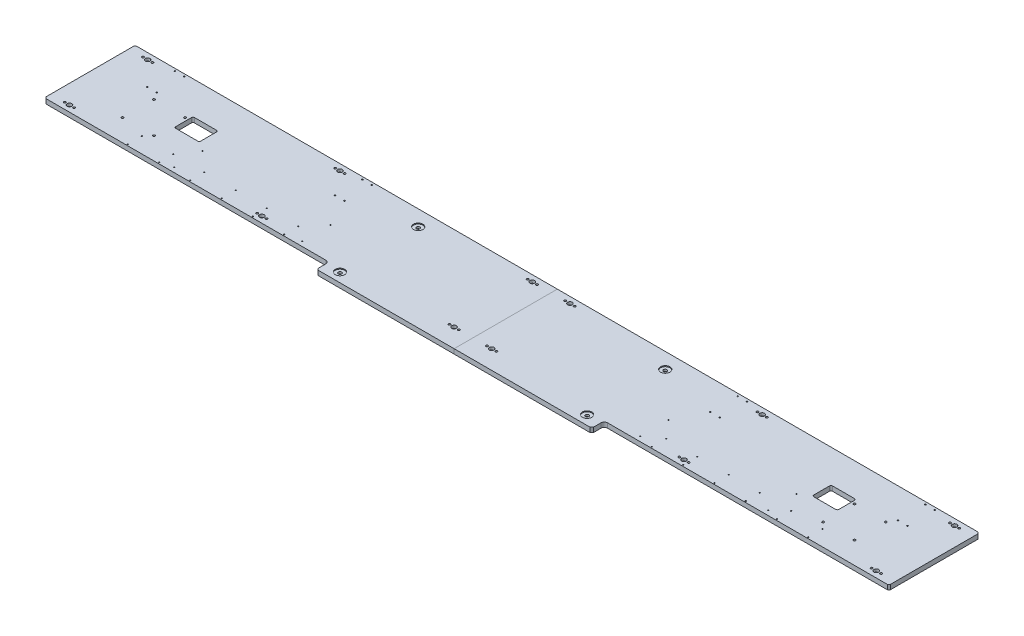
from build123d import *

# Parameters (mm, degrees)
SKETCH_1_W                = 2700
SKETCH_1_H                = 290
EXTRUDE_1_DEPTH           = 20
SKETCH_18_W               = 880
SKETCH_18_H               = 40
EXTRUDE_2_DEPTH           = 20
CHAMFER_1_SIZE            = 5
HOLE_WIZARD_1_D           = 9
HOLE_WIZARD_1_CBORE_D     = 15
HOLE_WIZARD_1_CBORE_DEPTH = 9
HOLE_WIZARD_M5_1_D        = 4.2
HOLE_WIZARD_M5_1_DEPTH    = 12.4
HOLE_WIZARD_M5_1_TIP      = 1.2618073
HOLE_WIZARD_M4_1_D        = 3.3
HOLE_WIZARD_M4_1_DEPTH    = 10.1
HOLE_WIZARD_M4_1_TIP      = 0.991420021
HOLE_WIZARD_M8_4_D        = 6.8
CUT_EXTRUDE_1_DEPTH       = 20
HOLE_WIZARD_3_D           = 11
HOLE_WIZARD_3_CBORE_D     = 18
HOLE_WIZARD_3_CBORE_DEPTH = 11
FILLET_1_R                = 10
HOLE_WIZARD_M8_2_D        = 6.8
SKETCH_21_R               = 15
CUT_EXTRUDE_2_DEPTH       = 3
HOLE_WIZARD_M4_2_D        = 3.3
HOLE_WIZARD_M4_2_DEPTH    = 10.1
HOLE_WIZARD_M4_2_TIP      = 0.991420021
SKETCH_25_W               = 2912.97775049
SKETCH_25_H               = 921.910734065
CUT_EXTRUDE_3_DEPTH       = 5


with BuildPart() as part:
    # 草图1 → 凸台-拉伸1 (new body)
    with BuildSketch(Plane(origin=(0, 0, 0), x_dir=(1, 0, 0), z_dir=(0, 1, 0))):
        Rectangle(SKETCH_1_W, SKETCH_1_H)
    extrude(amount=EXTRUDE_1_DEPTH)

    # 草图18 → 凸台-拉伸2 (add)
    with BuildSketch(Plane(origin=(0, 20, 0), x_dir=(1, 0, 0), z_dir=(0, 1, 0))):
        with Locations((0, -165)):
            Rectangle(SKETCH_18_W, SKETCH_18_H)
    extrude(amount=-EXTRUDE_2_DEPTH)

    # 倒角1
    chamfer_1_edges = [part.edges().sort_by_distance(p)[0] for p in [
        (-440, 10, 185),
        (440, 10, 185),
        (1350, 10, 145),
        (-1350, 10, 145),
        (-1350, 10, -145),
        (1350, 10, -145),
    ]]
    chamfer(chamfer_1_edges, length=CHAMFER_1_SIZE)

    # 打孔尺寸(%根据)内六角圆柱头螺钉的类型1 (through all)
    with Locations(Plane(origin=(0, 20, 0), x_dir=(1, 0, 0), z_dir=(0, 1, 0))):
        with Locations((-1290, -125), (-675, -125), (-60, -125), (-675, 125), (-60, 125), (-1290, 125), (1290, 125), (60, 125), (675, 125), (60, -125), (675, -125), (1290, -125)):
            CounterBoreHole(HOLE_WIZARD_1_D / 2, HOLE_WIZARD_1_CBORE_D / 2, HOLE_WIZARD_1_CBORE_DEPTH)

    # M5 螺纹孔1
    with Locations(Plane(origin=(0, 20, 0), x_dir=(1, 0, 0), z_dir=(0, 1, 0))):
        with Locations((-585, 49.25), (-615, 49.25), (-1185, 49.25), (-1215, 49.25), (-585, 136.75), (-615, 136.75), (-1185, 136.75), (-1215, 136.75), (1215, 136.75), (1185, 136.75), (615, 136.75), (585, 136.75), (1215, 49.25), (1185, 49.25), (615, 49.25), (585, 49.25)):
            Hole(HOLE_WIZARD_M5_1_D / 2, depth=HOLE_WIZARD_M5_1_DEPTH)
            with Locations((0, 0, -(HOLE_WIZARD_M5_1_DEPTH + HOLE_WIZARD_M5_1_TIP / 2))):  # 118° drill point
                Cone(0, HOLE_WIZARD_M5_1_D / 2, HOLE_WIZARD_M5_1_TIP, mode=Mode.SUBTRACT)

    # M4 螺纹孔1
    with Locations(Plane(origin=(0, 20, 0), x_dir=(1, 0, 0), z_dir=(0, 1, 0))):
        with Locations((539.999999898, -40), (950, -129.999999534), (539.999999898, -129.999999534), (950, -40), (-950, -40), (-539.999999898, -129.999999534), (-950, -129.999999534), (-539.999999898, -40)):
            Hole(HOLE_WIZARD_M4_1_D / 2, depth=HOLE_WIZARD_M4_1_DEPTH)
            with Locations((0, 0, -(HOLE_WIZARD_M4_1_DEPTH + HOLE_WIZARD_M4_1_TIP / 2))):  # 118° drill point
                Cone(0, HOLE_WIZARD_M4_1_D / 2, HOLE_WIZARD_M4_1_TIP, mode=Mode.SUBTRACT)

    # M8 螺纹孔4 (through all)
    with Locations(Plane(origin=(0, 20, 0), x_dir=(1, 0, 0), z_dir=(0, 1, 0))):
        with Locations((-1305, -125), (-1275, -125), (-690, -125), (-660, -125), (-75, -125), (-45, -125), (-690, 125), (-660, 125), (-75, 125), (-45, 125), (-1305, 125), (-1275, 125), (1275, 125), (1305, 125), (45, 125), (75, 125), (660, 125), (690, 125), (45, -125), (75, -125), (660, -125), (690, -125), (1275, -125), (1305, -125)):
            Hole(HOLE_WIZARD_M8_4_D / 2)

    # 草图11 → 切除-拉伸1 (cut)
    with BuildSketch(Plane(origin=(0, 20, 0), x_dir=(1, 0, 0), z_dir=(0, 1, 0))):
        with BuildLine():
            Line((-1055, 40), (-985, 40))
            ThreePointArc((-985, 40), (-981.464466094, 38.535533906), (-980, 35))
            Line((-980, 35), (-980, -15))
            ThreePointArc((-980, -15), (-981.464466094, -18.535533906), (-985, -20))
            Line((-985, -20), (-1055, -20))
            ThreePointArc((-1055, -20), (-1058.535533906, -18.535533906), (-1060, -15))
            Line((-1060, -15), (-1060, 35))
            ThreePointArc((-1060, 35), (-1058.535533906, 38.535533906), (-1055, 40))
        make_face()
        with BuildLine():
            Line((980, 35), (980, -15))
            ThreePointArc((980, -15), (981.464466094, -18.535533906), (985, -20))
            Line((985, -20), (1055, -20))
            ThreePointArc((1055, -20), (1058.535533906, -18.535533906), (1060, -15))
            Line((1060, -15), (1060, 35))
            ThreePointArc((1060, 35), (1058.535533906, 38.535533906), (1055, 40))
            Line((1055, 40), (985, 40))
            ThreePointArc((985, 40), (981.464466094, 38.535533906), (980, 35))
        make_face()
    extrude(amount=-CUT_EXTRUDE_1_DEPTH, mode=Mode.SUBTRACT)

    # 打孔尺寸(%根据)内六角圆柱头螺钉的类型3 (through all)
    with Locations(Plane(origin=(0, 0, 0), x_dir=(-1, 0, 0), z_dir=(0, -1, 0))):
        with Locations((395, -155), (395, 95), (-395, 95), (-395, -155)):
            CounterBoreHole(HOLE_WIZARD_3_D / 2, HOLE_WIZARD_3_CBORE_D / 2, HOLE_WIZARD_3_CBORE_DEPTH)

    # 圆角1
    fillet_1_edges = [part.edges().sort_by_distance(p)[0] for p in [
        (-440, 10, 145),
        (440, 10, 145),
    ]]
    fillet(fillet_1_edges, radius=FILLET_1_R)

    # M8 螺纹孔2 (through all)
    with Locations(Plane(origin=(0, 20, 0), x_dir=(1, 0, 0), z_dir=(0, 1, 0))):
        with Locations((1170, 25), (1070, 25), (1070, -75), (1170, -75), (-1170, -75), (-1070, -75), (-1070, 25), (-1170, 25)):
            Hole(HOLE_WIZARD_M8_2_D / 2)

    # 草图21 → 切除-拉伸2 (cut)
    with BuildSketch(Plane.XZ.offset(-20)):
        with Locations(Location((395, 155, 0), (0, 0, 270))):
            Circle(SKETCH_21_R)
        with Locations(Location((395, -95, 0), (0, 0, 270))):
            Circle(SKETCH_21_R)
        with Locations(Location((-395, -95, 0), (0, 0, 90))):
            Circle(SKETCH_21_R)
        with Locations(Location((-395, 155, 0), (0, 0, 90))):
            Circle(SKETCH_21_R)
    extrude(amount=CUT_EXTRUDE_2_DEPTH, mode=Mode.SUBTRACT)

    # M4 螺纹孔2
    with Locations(Plane(origin=(0, 20, 0), x_dir=(1, 0, 0), z_dir=(0, 1, 0))):
        with Locations((-1088, -95.5), (-1088, -140.5), (-988, -95.5), (-988, -140.5), (-888, -95.5), (-888, -140.5), (-788, -95.5), (-788, -140.5), (-688, -95.5), (-688, -140.5), (688, -140.5), (688, -95.5), (788, -140.5), (788, -95.5), (888, -140.5), (888, -95.5), (988, -140.5), (988, -95.5), (1088, -140.5), (1088, -95.5), (-588, -95.5), (-588, -140.5), (588, -140.5), (588, -95.5)):
            Hole(HOLE_WIZARD_M4_2_D / 2, depth=HOLE_WIZARD_M4_2_DEPTH)
            with Locations((0, 0, -(HOLE_WIZARD_M4_2_DEPTH + HOLE_WIZARD_M4_2_TIP / 2))):  # 118° drill point
                Cone(0, HOLE_WIZARD_M4_2_D / 2, HOLE_WIZARD_M4_2_TIP, mode=Mode.SUBTRACT)

    # 草图25 → 切除-拉伸3 (cut)
    with BuildSketch(Plane(origin=(0, 0, 0), x_dir=(-1, 0, 0), z_dir=(0, -1, 0))):
        with Locations((3.053578506, -64.770878484)):
            Rectangle(SKETCH_25_W, SKETCH_25_H)
    extrude(amount=-CUT_EXTRUDE_3_DEPTH, mode=Mode.SUBTRACT)


solid = part.part
